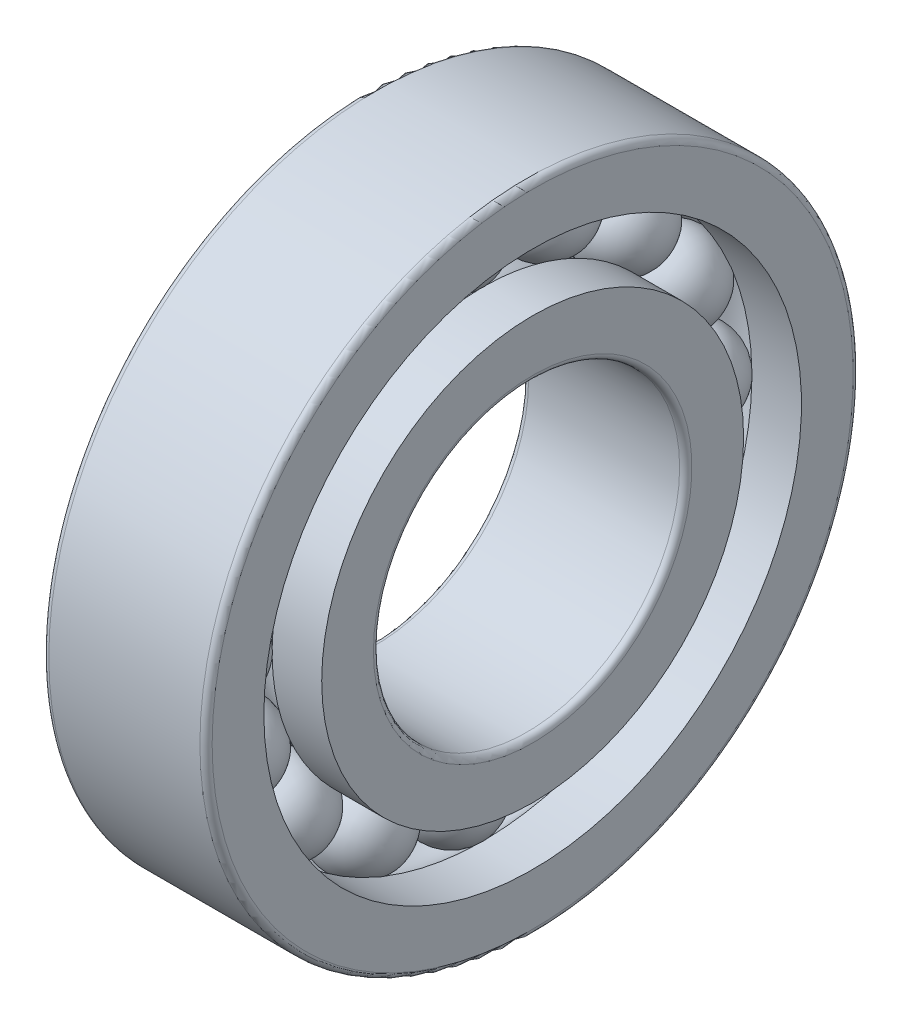
from build123d import *

# Parameters (mm, degrees)
CIRCULAR_PATTERN1_COUNT = 16
FILLET1_R               = 0.3


with BuildPart() as part:
    # Sketch1 → Revolve1 (revolve)
    with BuildSketch(Plane.XY):
        with BuildLine():
            Line((-2.125, 11.75), (2.125, 11.75))
            ThreePointArc((2.125, 11.75), (1.3e-16, 13.875), (-2.125, 11.75))
        make_face()
    revolve1 = revolve(axis=Axis((-4.596601835273904, 11.75, 0), (1, 0, 0)))

    # Sketch2 → Revolve2 (revolve)
    with BuildSketch(Plane.XY, mode=Mode.PRIVATE) as revolve2_sk:
        with BuildLine():
            Line((-4.000000000000001, 10.333333333333332), (-4.000000000000001, 7.5))
            Line((-4.000000000000001, 7.5), (4, 7.5))
            Line((4, 7.5), (4, 10.333333333333334))
            Line((4, 10.333333333333334), (1.5704396058287482, 10.333333333333334))
            ThreePointArc((1.5704396058287482, 10.333333333333334), (1.3e-16, 9.635000000000002), (-1.5704396058287482, 10.333333333333334))
            Line((-1.5704396058287482, 10.333333333333334), (-4.000000000000001, 10.333333333333332))
        make_face()
    revolve(revolve2_sk.sketch.rotate(Axis((-6.971390126215839, 0, 0), (1, 0, 0)), 90), axis=Axis((-6.971390126215839, 0, 0), (1, 0, 0)))

    # Sketch3 → Revolve3 (revolve)
    with BuildSketch(Plane.XY, mode=Mode.PRIVATE) as revolve3_sk:
        with BuildLine():
            Line((-4.000000000000002, 16), (3.9999999999999982, 16))
            Line((3.9999999999999982, 16), (3.9999999999999982, 13.166666666666666))
            Line((3.9999999999999982, 13.166666666666666), (1.5704396058287489, 13.166666666666666))
            ThreePointArc((1.5704396058287489, 13.166666666666666), (1.3e-16, 13.865), (-1.5704396058287489, 13.166666666666666))
            Line((-1.5704396058287489, 13.166666666666666), (-4.000000000000002, 13.166666666666666))
            Line((-4.000000000000002, 13.166666666666666), (-4.000000000000002, 16))
        make_face()
    revolve(revolve3_sk.sketch.rotate(Axis((-8.710676494715049, 0, 0), (1, 0, 0)), 90), axis=Axis((-8.710676494715049, 0, 0), (1, 0, 0)))

    # Circular-Pattern1: Revolve1 ×16 about axis
    circular_pattern1_axis = Axis((0, -1.3e-16, 2.1e-16), (1, 0, 0))
    for i in range(1, CIRCULAR_PATTERN1_COUNT):
        add(revolve1.rotate(circular_pattern1_axis, i * 360 / CIRCULAR_PATTERN1_COUNT))

    # Fillet1
    fillet1_edges = [part.edges().sort_by_distance(p)[0] for p in [
        (-4.000000000000002, -3.74e-15, -16),
        (3.9999999999999982, -3.74e-15, -16),
        (-4.000000000000001, -5.08e-15, -7.5),
        (4, -5.08e-15, -7.5),
    ]]
    fillet(fillet1_edges, radius=FILLET1_R)


solid = part.part
